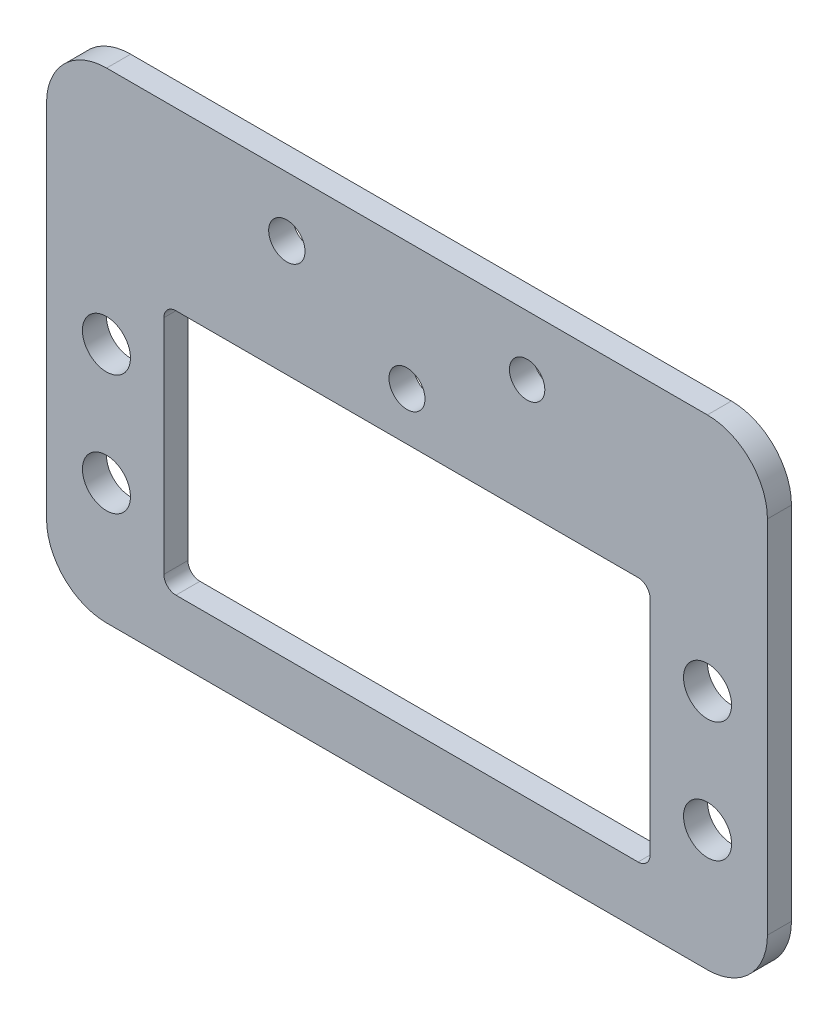
from build123d import *

# Parameters (mm, degrees)
BOSS_EXTRUDE1_DEPTH     = 2
CUT_EXTRUDE1_DEPTH      = 42.707695968
CUT_EXTRUDE1_DEPTH_BACK = 42.707695968
SKETCH3_R               = 1.5
SKETCH3_R_2             = 1.472115529
SKETCH3_R_3             = 1.512476654
CUT_EXTRUDE2_DEPTH      = 42.707695968
SKETCH4_R               = 2
CUT_EXTRUDE3_DEPTH      = 42.707695968


with BuildPart() as part:
    # Sketch1 → Boss-Extrude1 (new body)
    with BuildSketch(Plane.XY):
        with BuildLine():
            Line((-22.843450479, 26.485623003), (27.156549521, 26.485623003))
            ThreePointArc((27.156549521, 26.485623003), (30.692083427, 25.021156909), (32.156549521, 21.485623003))
            Line((32.156549521, 21.485623003), (32.156549521, -8.514376997))
            ThreePointArc((32.156549521, -8.514376997), (30.692083427, -12.049910903), (27.156549521, -13.514376997))
            Line((27.156549521, -13.514376997), (-22.843450479, -13.514376997))
            ThreePointArc((-22.843450479, -13.514376997), (-26.378984385, -12.049910903), (-27.843450479, -8.514376997))
            Line((-27.843450479, -8.514376997), (-27.843450479, 21.485623003))
            ThreePointArc((-27.843450479, 21.485623003), (-26.378984385, 25.021156909), (-22.843450479, 26.485623003))
        make_face()
    extrude(amount=BOSS_EXTRUDE1_DEPTH)

    # Sketch2 → Cut-Extrude1 (cut, two sides: drawn at the far end of the back side and taken through both)
    with BuildSketch(Plane.XY.offset(2).offset(-CUT_EXTRUDE1_DEPTH_BACK)):
        with BuildLine():
            Line((-17.075923419, 11.875959063), (21.38902246, 11.875959063))
            ThreePointArc((21.38902246, 11.875959063), (22.096129242, 11.583065844), (22.38902246, 10.875959063))
            Line((22.38902246, 10.875959063), (22.38902246, -7.624040937))
            ThreePointArc((22.38902246, -7.624040937), (22.096129242, -8.331147718), (21.38902246, -8.624040937))
            Line((21.38902246, -8.624040937), (-17.075923419, -8.624040937))
            ThreePointArc((-17.075923419, -8.624040937), (-17.7830302, -8.331147718), (-18.075923419, -7.624040937))
            Line((-18.075923419, -7.624040937), (-18.075923419, 10.875959063))
            ThreePointArc((-18.075923419, 10.875959063), (-17.7830302, 11.583065844), (-17.075923419, 11.875959063))
        make_face()
    extrude(amount=CUT_EXTRUDE1_DEPTH + CUT_EXTRUDE1_DEPTH_BACK, mode=Mode.SUBTRACT)

    # Sketch3 → Cut-Extrude2 (cut, through all)
    with BuildSketch(Plane.XY.offset(2)):
        with Locations((2.156549521, 15.875959063)):
            Circle(SKETCH3_R)
        with Locations((12.156549521, 21.525959063)):
            Circle(SKETCH3_R_2)
        with Locations((-7.843450479, 21.525959063)):
            Circle(SKETCH3_R_3)
    extrude(amount=-CUT_EXTRUDE2_DEPTH, mode=Mode.SUBTRACT)

    # Sketch4 → Cut-Extrude3 (cut, through all)
    with BuildSketch(Plane.XY.offset(2)):
        with Locations((27.17171292, -3.424040937)):
            Circle(SKETCH4_R)
        with Locations((27.17171292, 6.575959063)):
            Circle(SKETCH4_R)
        with Locations(Location((-22.858613878, -3.424040937, 0), (0, 0, 180))):
            Circle(SKETCH4_R)
        with Locations(Location((-22.858613878, 6.575959063, 0), (0, 0, 180))):
            Circle(SKETCH4_R)
    extrude(amount=-CUT_EXTRUDE3_DEPTH, mode=Mode.SUBTRACT)


solid = part.part
